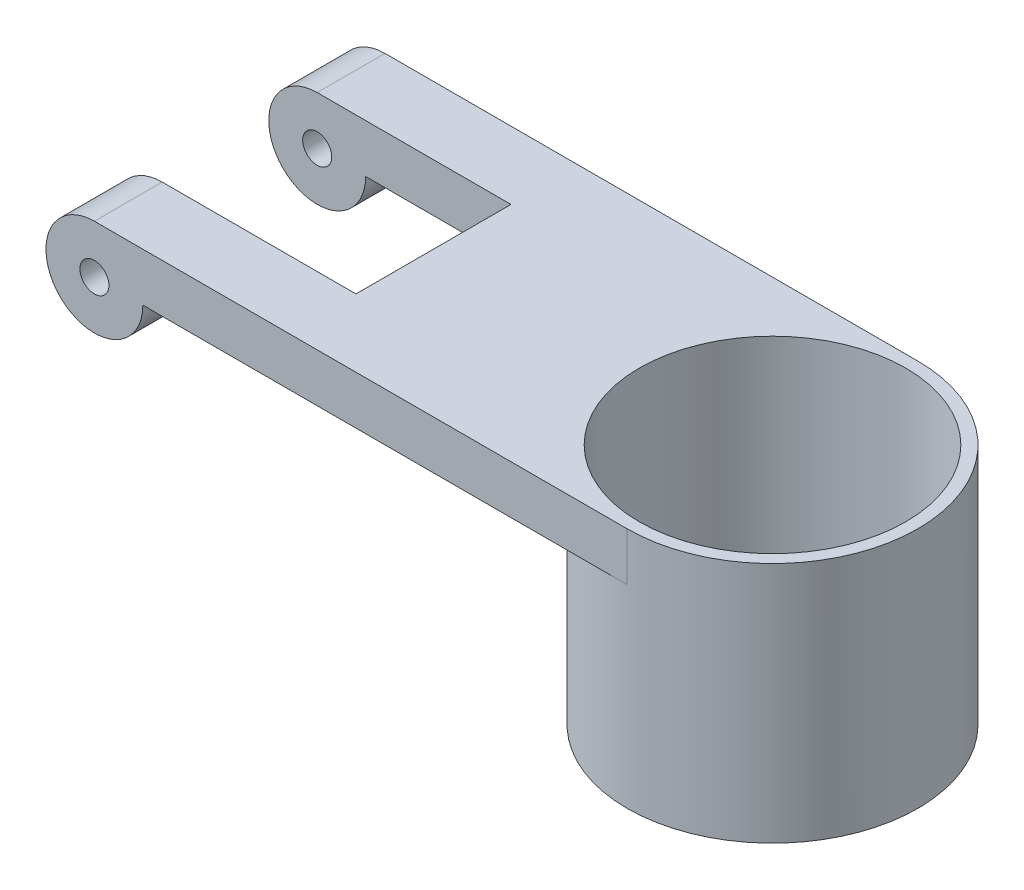
from build123d import *

# Parameters (mm, degrees)
SKETCH1_R               = 10
SKETCH1_R_2             = 3
BOSS_EXTRUDE1_DEPTH     = 60
BOSS_EXTRUDE2_START     = -60
BOSS_EXTRUDE2_DEPTH     = 60
CUT_EXTRUDE1_DEPTH      = 127.885775404
CUT_EXTRUDE1_DEPTH_BACK = 127.885775404
SKETCH4_W               = 97.330885133
SKETCH4_H               = 32
SKETCH5_R               = 30
SKETCH5_R_2             = 27.5
BOSS_EXTRUDE3_DEPTH     = 50
CUT_EXTRUDE2_DEPTH      = 161.312195419
CUT_EXTRUDE2_DEPTH_BACK = 161.312195419
SKETCH6_R               = 27.5


with BuildPart() as part:
    # Sketch1 → Boss-Extrude1 (new body)
    with BuildSketch(Plane.XY):
        Circle(SKETCH1_R)
        Circle(SKETCH1_R_2, mode=Mode.SUBTRACT)
    extrude(amount=BOSS_EXTRUDE1_DEPTH)

    # Sketch3 → Boss-Extrude2 (add)
    with BuildSketch(Plane.XY.offset(60).offset(BOSS_EXTRUDE2_START)):
        with BuildLine():
            Line((0, 10), (110, 10))
            Line((110, 10), (110, 0))
            Line((110, 0), (10, 0))
            ThreePointArc((10, 0), (7.071067812, 7.071067812), (0, 10))
        make_face()
    extrude(amount=BOSS_EXTRUDE2_DEPTH)

    # Sketch4 → Cut-Extrude1 (cut, two sides: drawn at the far end of the back side and taken through both)
    with BuildSketch(Plane(origin=(0, 10, 0), x_dir=(1, 0, 0), z_dir=(0, 1, 0)).offset(-CUT_EXTRUDE1_DEPTH_BACK)):
        with Locations((-8.665442567, -30)):
            Rectangle(SKETCH4_W, SKETCH4_H)
    extrude(amount=CUT_EXTRUDE1_DEPTH + CUT_EXTRUDE1_DEPTH_BACK, mode=Mode.SUBTRACT)

    # Sketch5 → Boss-Extrude3 (add)
    with BuildSketch(Plane(origin=(0, 10, 0), x_dir=(1, 0, 0), z_dir=(0, 1, 0))):
        with Locations(Location((110, -30, 0), (0, 0, 270))):
            Circle(SKETCH5_R)
        with Locations(Location((110, -30, 0), (0, 0, 270))):
            Circle(SKETCH5_R_2, mode=Mode.SUBTRACT)
    extrude(amount=-BOSS_EXTRUDE3_DEPTH)

    # Sketch6 → Cut-Extrude2 (cut, two sides: drawn at the far end of the back side and taken through both)
    with BuildSketch(Plane(origin=(0, 10, 0), x_dir=(1, 0, 0), z_dir=(0, 1, 0)).offset(-CUT_EXTRUDE2_DEPTH_BACK)):
        with Locations(Location((110, -30, 0), (0, 0, 270))):
            Circle(SKETCH6_R)
    extrude(amount=CUT_EXTRUDE2_DEPTH + CUT_EXTRUDE2_DEPTH_BACK, mode=Mode.SUBTRACT)


solid = part.part
